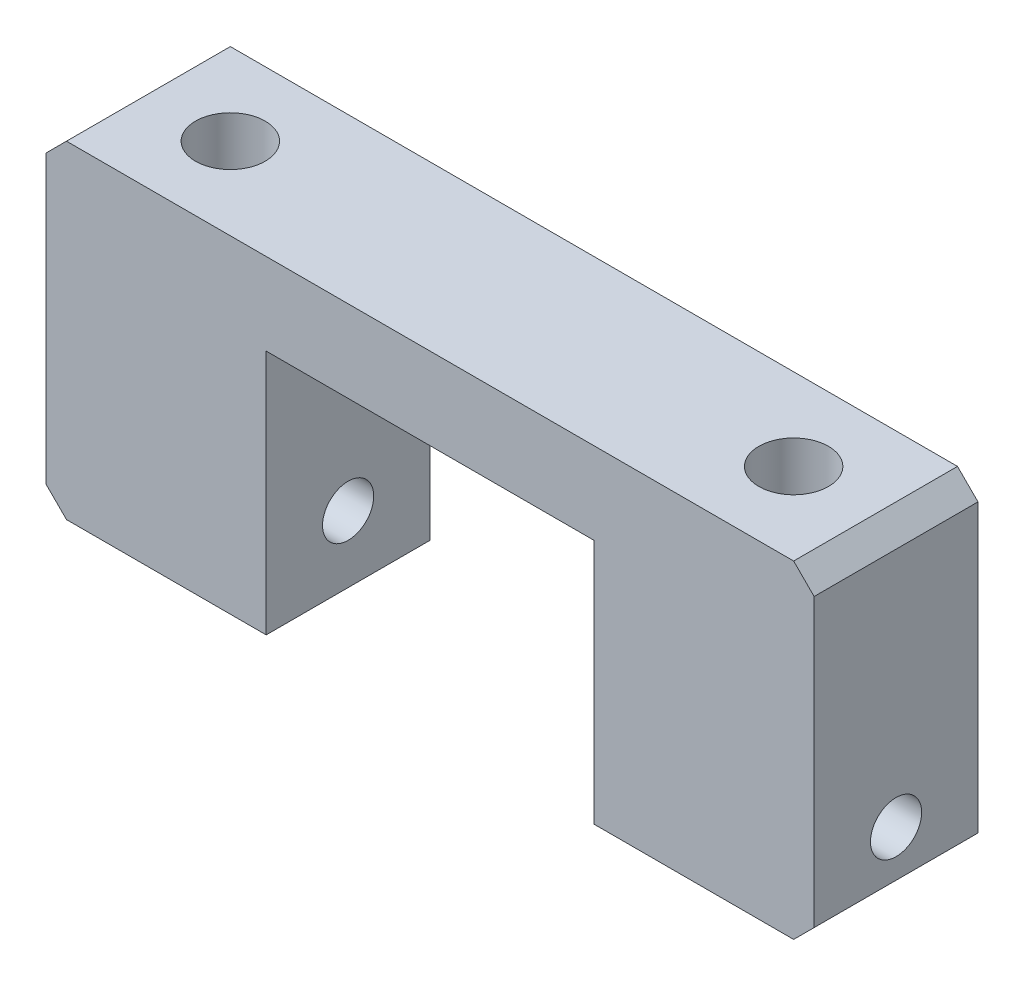
from build123d import *

# Parameters (mm, degrees)
SKETCH_1_W             = 75
SKETCH_1_H             = 32
EXTRUDE_1_DEPTH        = 8
SKETCH_3_W             = 32
SKETCH_3_H             = 24
CUT_EXTRUDE_1_DEPTH    = 44.797830997
HOLE_WIZARD_M6_1_D     = 5
CHAMFER_1_SIZE         = 2
HOLE_WIZARD_M8_1_D     = 6.8
HOLE_WIZARD_M8_1_DEPTH = 19.75
HOLE_WIZARD_M8_1_TIP   = 2.042926105
CHAMFER_2_SIZE         = 2


with BuildPart() as part:
    # 草图1 → 凸台-拉伸1 (new, symmetric)
    with BuildSketch(Plane.XY):
        Rectangle(SKETCH_1_W, SKETCH_1_H)
    extrude(amount=EXTRUDE_1_DEPTH, both=True)

    # 草图3 → 切除-拉伸1 (cut, through all)
    with BuildSketch(Plane.XY.offset(8)):
        with Locations((0, -4)):
            Rectangle(SKETCH_3_W, SKETCH_3_H)
    extrude(amount=-CUT_EXTRUDE_1_DEPTH, mode=Mode.SUBTRACT)

    # M6 螺纹孔1 (through all)
    with Locations(Plane(origin=(37.5, 0, 0), x_dir=(0, 0, -1), z_dir=(1, 0, 0))):
        with Locations((0, -9.5)):
            Hole(HOLE_WIZARD_M6_1_D / 2)

    # 倒角1
    chamfer_1_edges = [part.edges().sort_by_distance(p)[0] for p in [
        (-37.5, 16, 0),
        (37.5, 16, 0),
    ]]
    chamfer(chamfer_1_edges, length=CHAMFER_1_SIZE)

    # M8 螺纹孔1
    with Locations(Plane(origin=(0, 16, 0), x_dir=(1, 0, 0), z_dir=(0, 1, 0))):
        with Locations((-27.5, 0), (27.5, 0)):
            Hole(HOLE_WIZARD_M8_1_D / 2, depth=HOLE_WIZARD_M8_1_DEPTH)
            with Locations((0, 0, -(HOLE_WIZARD_M8_1_DEPTH + HOLE_WIZARD_M8_1_TIP / 2))):  # 118° drill point
                Cone(0, HOLE_WIZARD_M8_1_D / 2, HOLE_WIZARD_M8_1_TIP, mode=Mode.SUBTRACT)

    # 倒角2
    chamfer_2_edges = [part.edges().sort_by_distance(p)[0] for p in [
        (37.5, -16, 0),
        (-37.5, -16, 0),
    ]]
    chamfer(chamfer_2_edges, length=CHAMFER_2_SIZE)


solid = part.part
